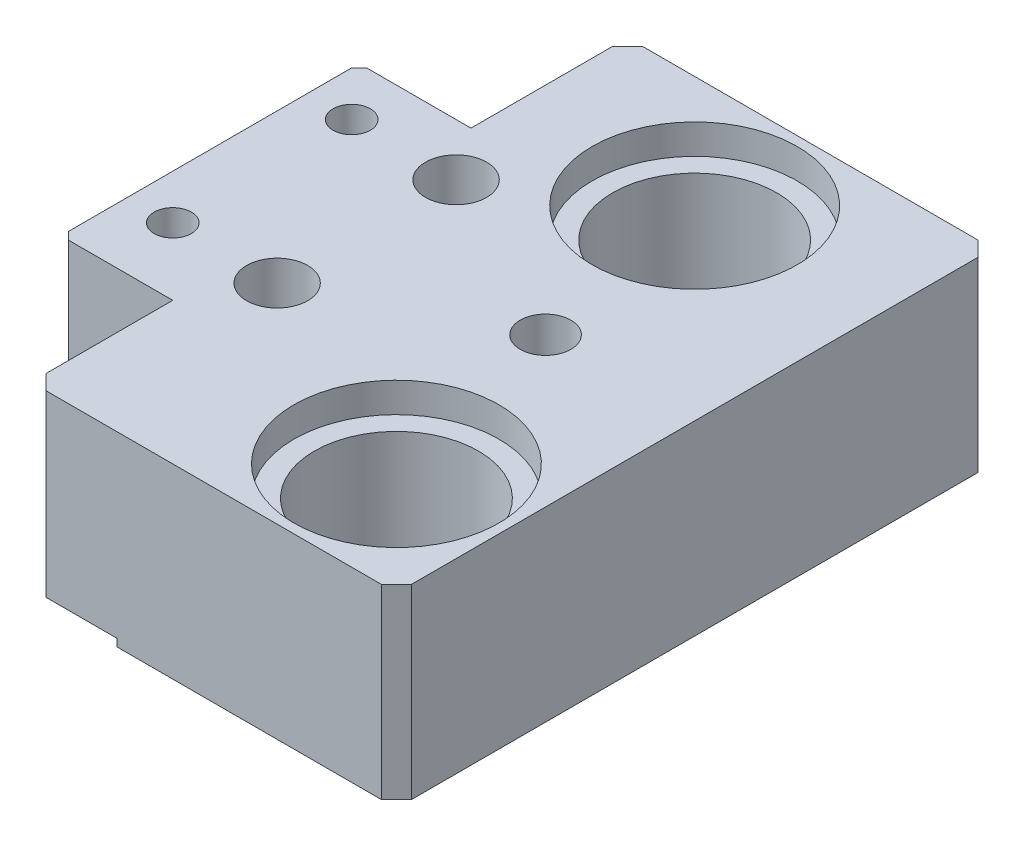
from build123d import *

# Parameters (mm, degrees)
SKETCH1_W             = 64
SKETCH1_H             = 25
BOSS_EXTRUDE1_DEPTH   = 40
SKETCH3_R             = 11
SKETCH3_R_2           = 2.5
CUT_EXTRUDE1_DEPTH    = 58
M3_TAPPED_HOLE1_D     = 2.5
M3_TAPPED_HOLE1_DEPTH = 7.5
M3_TAPPED_HOLE1_TIP   = 0.751075774
M8_TAPPED_HOLE1_D     = 6.8
M8_TAPPED_HOLE1_DEPTH = 20
M8_TAPPED_HOLE1_TIP   = 2.042926105
SKETCH11_W            = 15
SKETCH11_H            = 21
SKETCH11_H_2          = 19
CUT_EXTRUDE5_DEPTH    = 58
SKETCH13_R            = 4
SKETCH13_R_2          = 4.1
CUT_EXTRUDE7_DEPTH    = 13
SKETCH14_R            = 4.1
CUT_EXTRUDE8_DEPTH    = 6
SKETCH15_W            = 11.5
SKETCH15_H            = 80
CUT_EXTRUDE11_DEPTH   = 1
SKETCH16_R            = 13.75
CUT_EXTRUDE12_DEPTH   = 4
CHAMFER2_SIZE         = 2
CHAMFER3_SIZE         = 1


with BuildPart() as part:
    # Sketch1 → Boss-Extrude1 (new, symmetric)
    with BuildSketch(Plane.XY):
        Rectangle(SKETCH1_W, SKETCH1_H)
    extrude(amount=BOSS_EXTRUDE1_DEPTH, both=True)

    # Sketch3 → Cut-Extrude1 (cut, through all)
    with BuildSketch(Plane(origin=(0, 12.5, 0), x_dir=(1, 0, 0), z_dir=(0, 1, 0))):
        with Locations(Location((7, 25, 0), (0, 0, 180))):
            Circle(SKETCH3_R)
        with Locations(Location((17, -25, 0), (0, 0, 180))):
            Circle(SKETCH3_R)
        with Locations(Location((-12, 12, 0), (0, 0, 180))):
            Circle(SKETCH3_R_2)
        with Locations(Location((-12, -12, 0), (0, 0, 180))):
            Circle(SKETCH3_R_2)
        with Locations(Location((-26, 12, 0), (0, 0, 180))):
            Circle(SKETCH3_R_2)
        with Locations(Location((-26, -12, 0), (0, 0, 180))):
            Circle(SKETCH3_R_2)
    extrude(amount=-CUT_EXTRUDE1_DEPTH, mode=Mode.SUBTRACT)

    # M3 Tapped Hole1
    with Locations(Plane.ZY.offset(32)):
        with Locations((0, 3.5), (-6, -7.5), (6, -7.5)):
            Hole(M3_TAPPED_HOLE1_D / 2, depth=M3_TAPPED_HOLE1_DEPTH)
            with Locations((0, 0, -(M3_TAPPED_HOLE1_DEPTH + M3_TAPPED_HOLE1_TIP / 2))):  # 118° drill point
                Cone(0, M3_TAPPED_HOLE1_D / 2, M3_TAPPED_HOLE1_TIP, mode=Mode.SUBTRACT)

    # M8 Tapped Hole1
    with Locations(Plane(origin=(0, 12.5, 0), x_dir=(-1, 0, 0), z_dir=(0, 1, 0))):
        with Locations((-12, 0)):
            Hole(M8_TAPPED_HOLE1_D / 2, depth=M8_TAPPED_HOLE1_DEPTH)
            with Locations((0, 0, -(M8_TAPPED_HOLE1_DEPTH + M8_TAPPED_HOLE1_TIP / 2))):  # 118° drill point
                Cone(0, M8_TAPPED_HOLE1_D / 2, M8_TAPPED_HOLE1_TIP, mode=Mode.SUBTRACT)

    # Sketch11 → Cut-Extrude5 (cut, through all)
    with BuildSketch(Plane(origin=(0, 12.5, 0), x_dir=(1, 0, 0), z_dir=(0, 1, 0))):
        with Locations((-24.5, 29.5)):
            Rectangle(SKETCH11_W, SKETCH11_H)
        with Locations((-24.5, -30.5)):
            Rectangle(SKETCH11_W, SKETCH11_H_2)
    extrude(amount=-CUT_EXTRUDE5_DEPTH, mode=Mode.SUBTRACT)

    # Sketch13 → Cut-Extrude7 (cut)
    with BuildSketch(Plane.XZ.offset(12.5)):
        with Locations((-26, -12)):
            Circle(SKETCH13_R)
        with Locations((-26, 12)):
            Circle(SKETCH13_R)
        with Locations((-12, 12)):
            Circle(SKETCH13_R)
        with Locations((-12, -12)):
            Circle(SKETCH13_R)
        with Locations((-26, 0)):
            Circle(SKETCH13_R_2)
    extrude(amount=-CUT_EXTRUDE7_DEPTH, mode=Mode.SUBTRACT)

    # Sketch14 → Cut-Extrude8 (cut)
    with BuildSketch(Plane(origin=(0, 12.5, 0), x_dir=(1, 0, 0), z_dir=(0, 1, 0))):
        with Locations(Location((-12, -12, 0), (0, 0, 180))):
            Circle(SKETCH14_R)
        with Locations(Location((-12, 12, 0), (0, 0, 180))):
            Circle(SKETCH14_R)
    extrude(amount=-CUT_EXTRUDE8_DEPTH, mode=Mode.SUBTRACT)

    # Sketch15 → Cut-Extrude11 (cut)
    with BuildSketch(Plane(origin=(0, -12.5, 0), x_dir=(-1, 0, 0), z_dir=(0, -1, 0))):
        with Locations((11.25, 0)):
            Rectangle(SKETCH15_W, SKETCH15_H)
    extrude(amount=-CUT_EXTRUDE11_DEPTH, mode=Mode.SUBTRACT)

    # Sketch16 → Cut-Extrude12 (cut)
    with BuildSketch(Plane(origin=(0, 12.5, 0), x_dir=(1, 0, 0), z_dir=(0, 1, 0))):
        with Locations(Location((17, -25, 0), (0, 0, 180))):
            Circle(SKETCH16_R)
        with Locations(Location((7, 25, 0), (0, 0, 180))):
            Circle(SKETCH16_R)
    extrude(amount=-CUT_EXTRUDE12_DEPTH, mode=Mode.SUBTRACT)

    # Chamfer2
    chamfer2_edges = [part.edges().sort_by_distance(p)[0] for p in [
        (-17, 0.5, 40),
        (-17, 0.5, -40),
        (32, 0, 40),
        (32, 0, -40),
    ]]
    chamfer(chamfer2_edges, length=CHAMFER2_SIZE)

    # Chamfer3
    chamfer3_edges = [part.edges().sort_by_distance(p)[0] for p in [
        (-32, 0, -19),
        (-32, 0, 21),
    ]]
    chamfer(chamfer3_edges, length=CHAMFER3_SIZE)


solid = part.part
